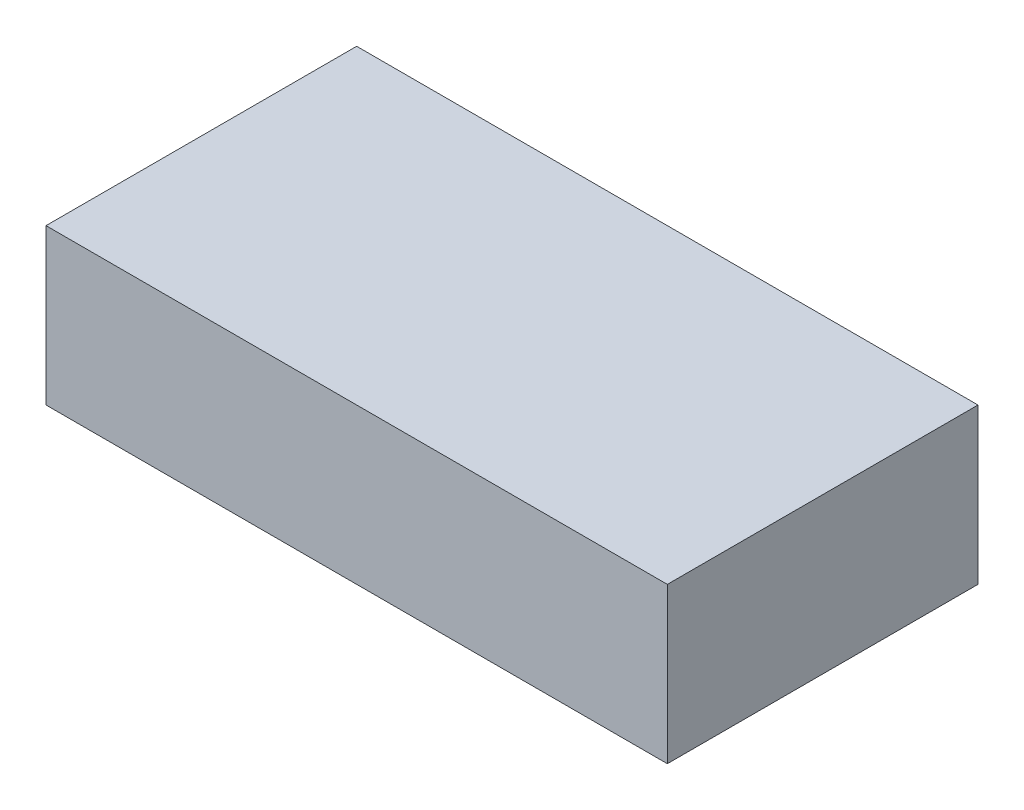
SolidWorks part; units mm, degrees
material "Q235B"
ref_plane "Front Plane" through (0, 0, 0) normal (0, 0, 1) x (1, 0, 0)
ref_plane "Top Plane" through (0, 0, 0) normal (0, 1, 0) x (1, 0, 0)
ref_plane "Right Plane" through (0, 0, 0) normal (1, 0, 0) x (0, 0, -1)
other "Configuration Table"
sketch "Sketch1" plane through (0, 0, 0) normal (0, 1, 0) x (1, 0, 0)
  line L1 (-10, -5) -> (10, -5)
  line L2 (-10, -5) -> (-10, 5)
  line L3 (-10, 5) -> (10, 5)
  line L4 (10, -5) -> (10, 5)
  line L5 (-10, -5) -> (10, 5) construction
  line L6 (-10, 5) -> (10, -5) construction
  point P0 (0, 0)
  dimension "D1" = 20
  dimension "D2" = 10
extrude "Boss-Extrude1" add sketch "Sketch1" along normal blind 5
